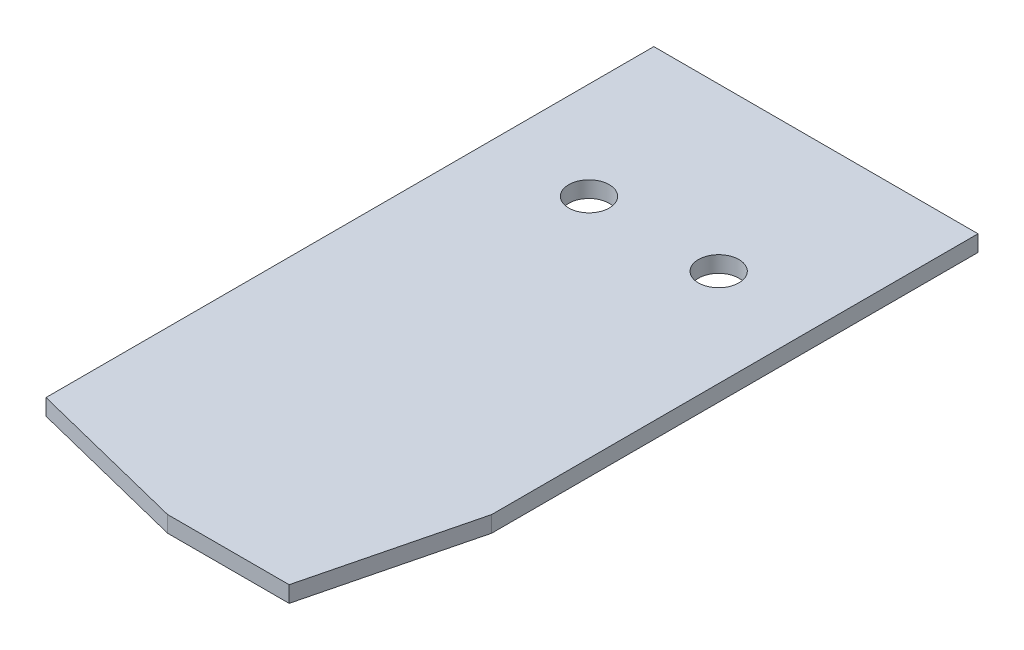
from build123d import *
from OCP.BRepFilletAPI import BRepFilletAPI_MakeChamfer

# Parameters (mm, degrees)
SKETCH1_W           = 40
SKETCH1_H           = 80
BOSS_EXTRUDE1_DEPTH = 2
SKETCH2_R           = 2.5
CUT_EXTRUDE1_DEPTH  = 10
CHAMFER1_SIZE       = 5
CHAMFER1_SIZE2      = 20


with BuildPart() as part:
    # Sketch1 → Boss-Extrude1 (new body)
    with BuildSketch(Plane(origin=(0, 0, 0), x_dir=(1, 0, 0), z_dir=(0, 1, 0))):
        Rectangle(SKETCH1_W, SKETCH1_H)
    extrude(amount=BOSS_EXTRUDE1_DEPTH)

    # Sketch2 → Cut-Extrude1 (cut)
    with BuildSketch(Plane.XZ):
        with Locations(Location((8, -20, 0), (0, 0, 270))):
            Circle(SKETCH2_R)
        with Locations(Location((-8, -20, 0), (0, 0, 270))):
            Circle(SKETCH2_R)
    extrude(amount=-CUT_EXTRUDE1_DEPTH, mode=Mode.SUBTRACT)

    # Chamfer1: one chamfer whose edges measure the first distance from different faces: ONE call of the kernel's chamfer builder (chamfer() names one face for all edges)
    chamfer1_edges_1 = [part.edges().sort_by_distance(p)[0] for p in [
        (20, 1, 40),
    ]]
    chamfer1_side_1 = [part.faces().sort_by_distance(p)[0] for p in [
        (0, 1, 40),
    ]]
    chamfer1_edges_2 = [part.edges().sort_by_distance(p)[0] for p in [
        (-20, 1, 40),
    ]]
    chamfer1_side_2 = [part.faces().sort_by_distance(p)[0] for p in [
        (-20, 1, 0),
    ]]
    chamfer1 = BRepFilletAPI_MakeChamfer(part.part.solid().wrapped)
    for e in chamfer1_edges_1:
        chamfer1.Add(CHAMFER1_SIZE, CHAMFER1_SIZE2, e.wrapped, chamfer1_side_1[0].wrapped)  # the first distance lies on this face
    for e in chamfer1_edges_2:
        chamfer1.Add(CHAMFER1_SIZE, CHAMFER1_SIZE2, e.wrapped, chamfer1_side_2[0].wrapped)  # the first distance lies on this face
    add(Compound.cast(chamfer1.Shape()), mode=Mode.REPLACE)


solid = part.part
